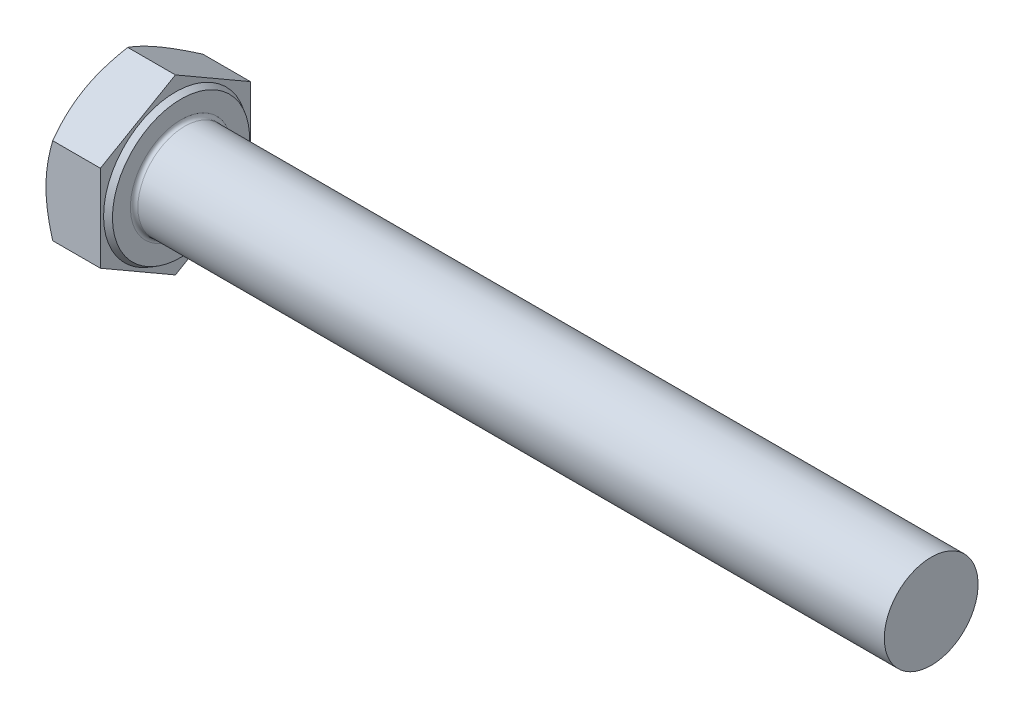
from build123d import *

# Parameters (mm, degrees)
EXTRUDE_384_DEPTH = 6.4
FILLET_1305_R     = 0.4


with BuildPart() as part:
    # 草图1 → Extrude 384 (new body)
    with BuildSketch(Plane(origin=(0, 0, 0), x_dir=(0, 0, -1), z_dir=(1, 0, 0))):
        Polygon((8, 4.618802154), (8, -4.618802154), (0, -9.237604307), (-8, -4.618802154), (-8, 4.618802154), (0, 9.237604307), align=None)
    extrude(amount=EXTRUDE_384_DEPTH)

    # 草图2 → 凸台-旋转1 (revolve)
    with BuildSketch(Plane.XY, mode=Mode.PRIVATE) as revolve_1_sk:
        Polygon((0, 0), (86.4, 0), (86.4, 3.701), (86.4, 5), (60.4, 5), (0, 5), align=None)
    revolve(revolve_1_sk.sketch.rotate(Axis((0, 0, 0), (1, 0, 0)), 90), axis=Axis((0, 0, 0), (1, 0, 0)))

    # 草图3 → 切除-旋转1 (revolve, cut)
    with BuildSketch(Plane.XY):
        Polygon((0, 8), (3.601282526, 14.237604307), (3.601282526, 19.237604307), (-10, 19.237604307), (-10, 8), align=None)
    revolve(axis=Axis((0, 0, 0), (1, 0, 0)), mode=Mode.SUBTRACT)

    # 草图4 → 切除-旋转3 (revolve, cut)
    with BuildSketch(Plane.XY, mode=Mode.PRIVATE) as cut_revolve_3_sk:
        Polygon((6.4, 7.315), (5.8, 7.661410162), (5.8, 9.237604307), (6.4, 9.237604307), align=None)
    revolve(cut_revolve_3_sk.sketch.rotate(Axis((0, 0, 0), (1, 0, 0)), 90), axis=Axis((0, 0, 0), (1, 0, 0)), mode=Mode.SUBTRACT)

    # Fillet 1305
    fillet_1305_edges = [part.edges().sort_by_distance(p)[0] for p in [
        (6.4, 0, -5),
    ]]
    fillet(fillet_1305_edges, radius=FILLET_1305_R)


solid = part.part
